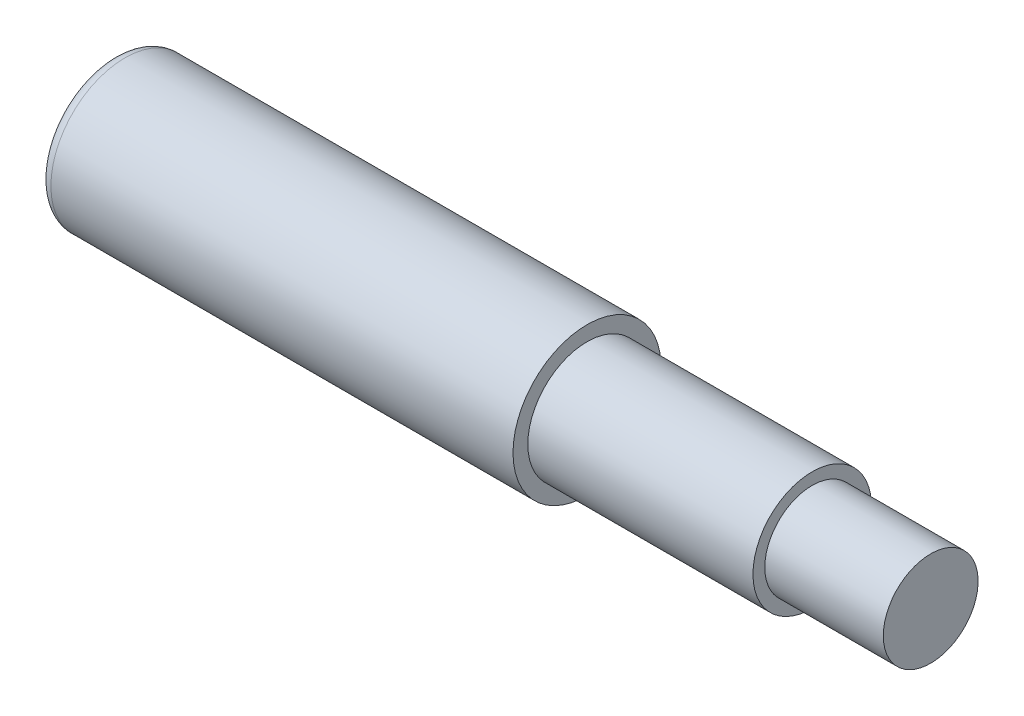
SolidWorks part; units mm, degrees
material "Q235A"
ref_plane "Front Plane" through (0, 0, 0) normal (0, 0, 1) x (1, 0, 0)
ref_plane "Top Plane" through (0, 0, 0) normal (0, 1, 0) x (1, 0, 0)
ref_plane "Right Plane" through (0, 0, 0) normal (1, 0, 0) x (0, 0, -1)
sketch "Sketch3" plane through (0, 0, 0) normal (0, 0, 1) x (1, 0, 0)
  line L0 (0, 0) -> (136.8406, 0) construction
  line L1 (0, 0) -> (0, 12.5)
  line L2 (0, 12.5) -> (80, 12.5)
  line L3 (80, 12.5) -> (80, 10)
  line L4 (80, 10) -> (118, 10)
  line L5 (118, 10) -> (118, 8)
  line L6 (118, 8) -> (138, 8)
  line L7 (138, 8) -> (138, 0)
  line L8 (0, 0) -> (138, 0)
  dimension "D1" = 25
  dimension "D2" = 20
  dimension "D3" = 16
  dimension "D4" = 80
  dimension "D5" = 38
  dimension "D6" = 20
revolve "Revolve1" add sketch "Sketch3" angle 360 about L0
fillet "Fillet1" radius 2 1 edges at (0, 0, 12.5)
